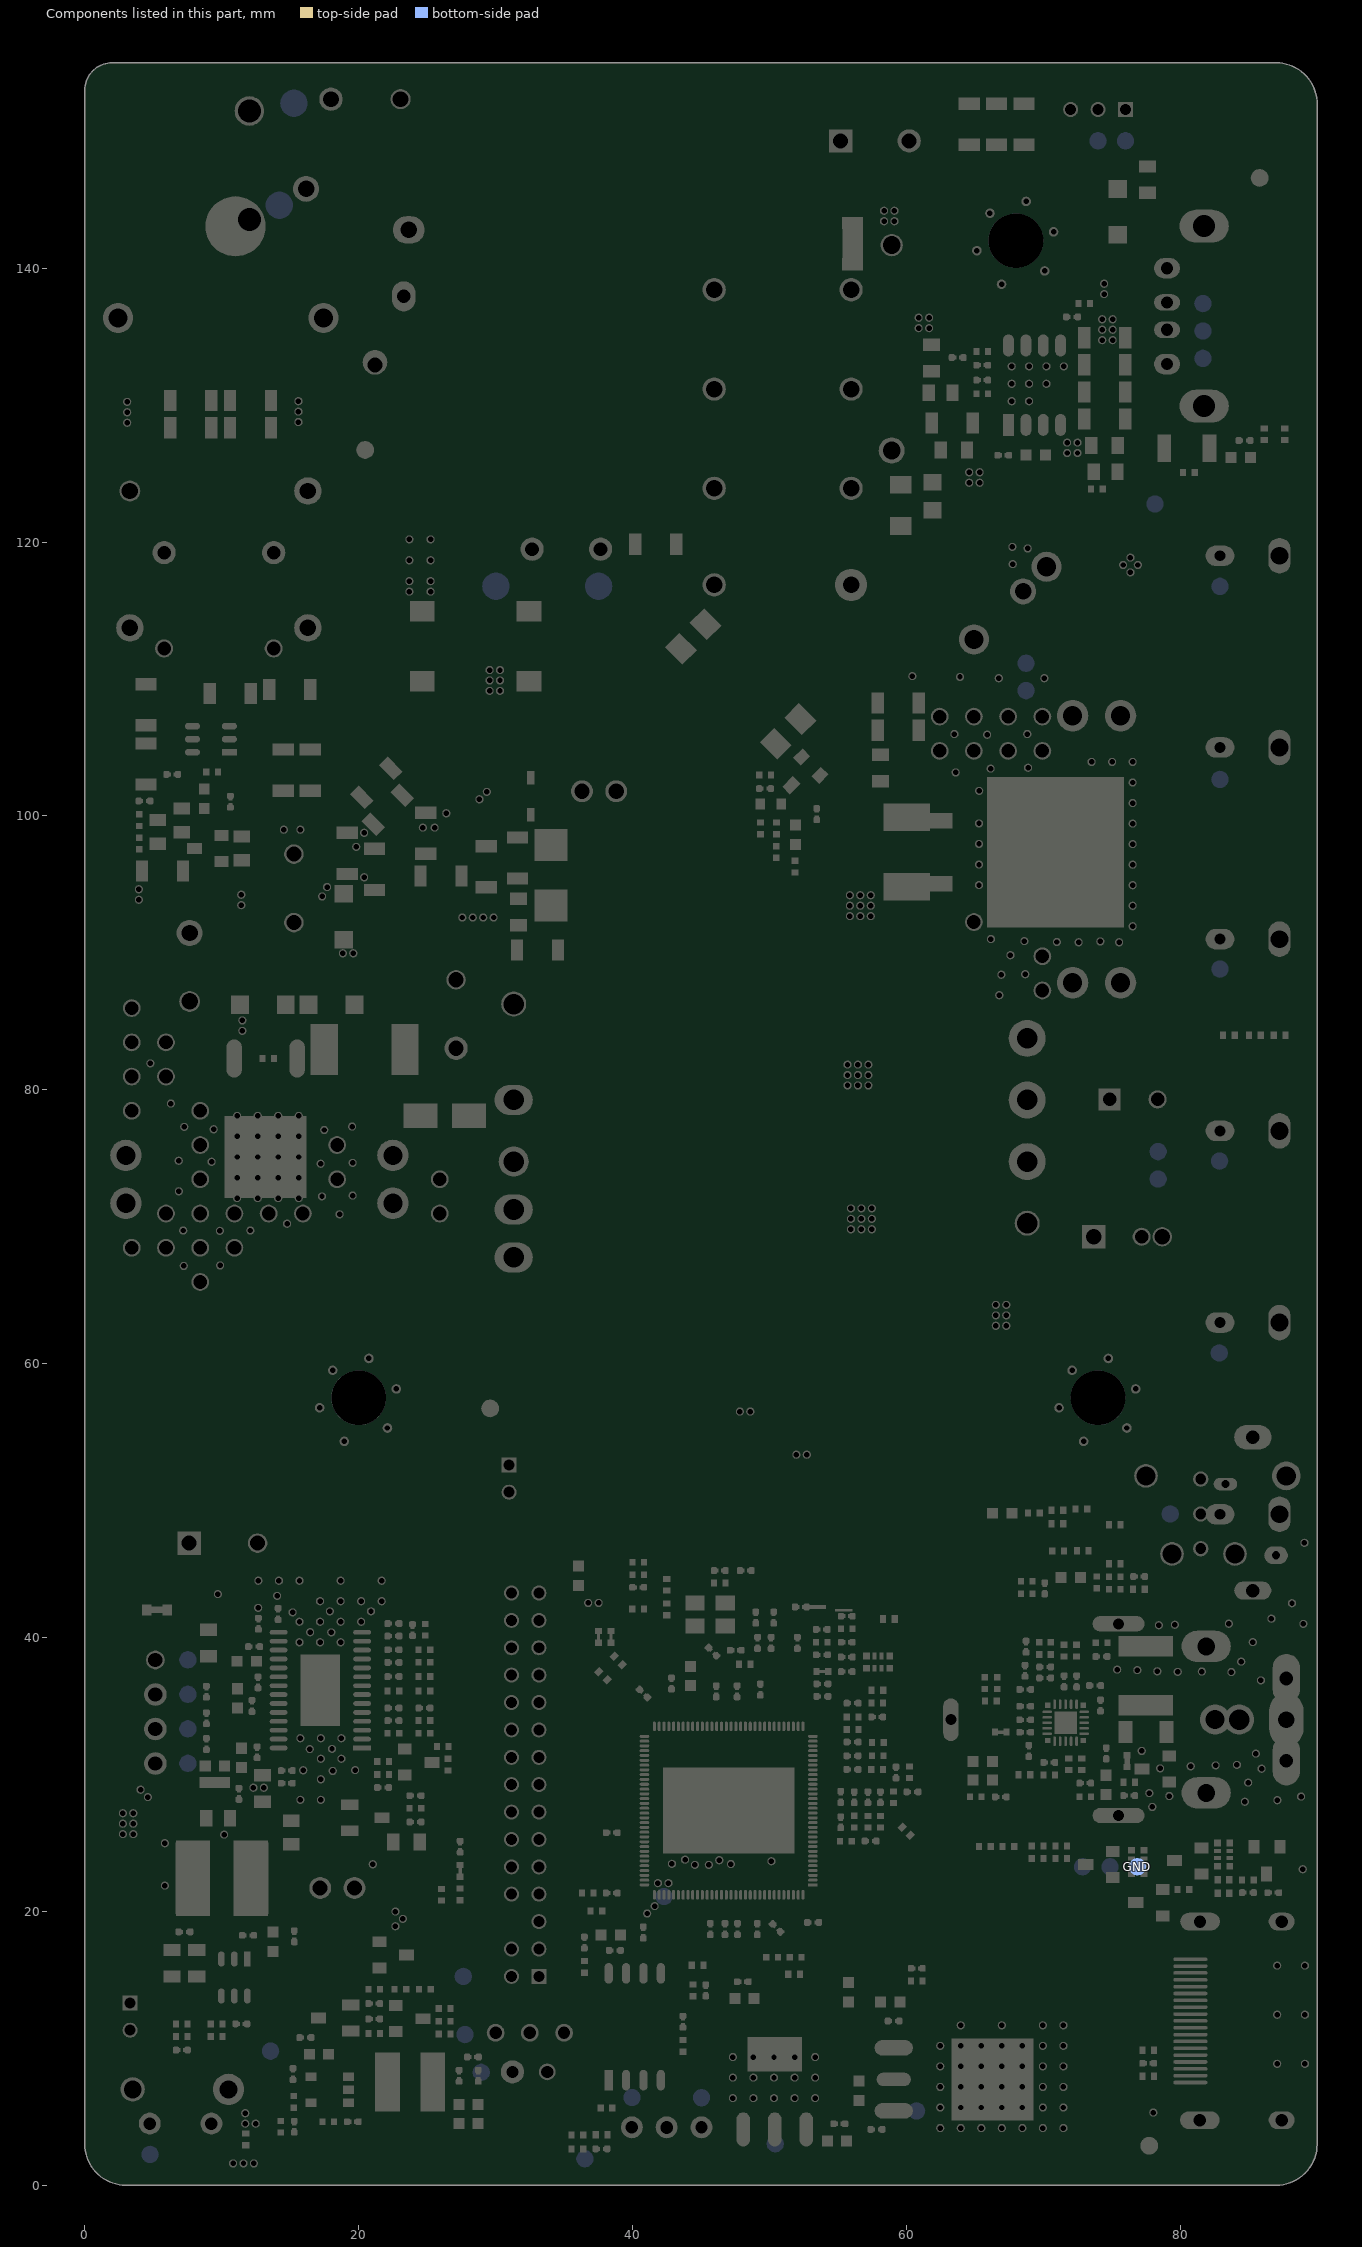
[diagram p0: the components of this part, seen from the top]
# Altium PCB MISC116569.PcbDoc (part 13 of 15)
Units mm, origin at the board's own origin, x right, y up, seen from the top; angles counter-clockwise.
Board outline 90 x 155 mm, 2 copper layers (TopLayer, BottomLayer), stack 1.571 mm thick; 527 components, 277 nets, 2450 pads, 649 vias.

## Via types
v1: diameter 0.6, hole 0.4, TopLayer to BottomLayer, tented both sides, 649 vias

## Nets (pads, with @x,y where several pads share a name; then routed paths per layer and width w, separated by ;. In a path a pad name is that pad's centre, name@x,y a point inside that pad or via, vN(x,y) a via of type N, cw(c..) or ccw(c..) an arc to the next point about the centre after c; other vN are vias at no path point) (continued)
pads on no net: "Conformal Coating.0" AV20.0 AV20.1@79.04,135.5 AV20.2@79.04,137.5 AV41.0 AV41.8 AVI1.0 AVI2.0 AVI3.0 AVO2.0 AVO3.0 AVO4.0 BOE.0 CA3.2@24.804,34.849 CA4.2@23.935,40.538 CA5.2@22.539,33.929 CA6.2@22.539,34.849 CA7.2@22.539,37.145 CA8.2@22.539,38.177 CA9.2@22.539,39.107 CA10.2@22.539,40.101 CA11.2@22.539,41.018 CA12.2@14.752,29.357 CA13.2@14.752,30.274 CA14.2@12.586,31.619 CA15.2@12.205,34.997 CA16.2@12.649,36.722 CA17.2@12.361,39.332 CA18.2@14.122,41.715 CA19.2@12.675,41.002 CA24.2@11.252,28.581 CA25.2@8.877,32.22 CA26.2@8.877,34.095 CA27.2@8.878,36.039 CA33.2@40.41,43.665 CB101.2@6.382,103.035 CB103.2@10.63,101.041 CB110.2@53.454,100.133 CB111.2@4.36,101.098 CB114.1@15.269,92.209 CB114.1@15.269,97.209 CB116.0 CB120.41 CB120.42 CB125.2@49.678,101.994 CB804.2@72.098,136.449 CB805.2@63.745,133.477 CB806.2@65.54,131.826 CB807.2@67.077,126.34 CB812.2@65.54,132.918 CD3.2@7.276,18.504 CD4.2@11.921,18.25 CD5.2@7.088,9.868 CD6.2@15.299,18.174 CD8.2@19.574,4.638 CD9.2@11.434,11.786 CD12.2@15.299,4.27 CD13.2@27.338,7.991 CD17.2@15.197,8.118 CF1.2@45.846,38.965 CF2.2@38.713,17.147 CF4.2@47.535,39.068 CF7.2@38.482,25.745 CF8.2@47.666,18.708 CF9.2@40.8,35.918 CF10.2@55.207,28.355 CF11.2@55.207,26.505 CF12.2@49.335,36.197 CF13.2@56.07,35.204 CF14.2@47.638,36.066 CF16.2@40.787,18.456 CF17.2@46.114,36.066 CF18.2@45.683,18.708 CF19.2@42.85,36.644 CF20.2@53.187,19.192 CF21.2@46.749,18.708 CF24.2@50.525,18.792 CF25.2@49.112,18.708 CF26.2@56.07,32.36 CF27.2@53.868,36.614 CF28.2@53.868,35.7 CF29.2@52.04,39.605 CF30.2@52.294,42.23 CF31.2@58.102,28.334 CF38.2@46.376,44.884 CF40.2@48.274,44.884 CG201.2@27.414,24.719 CH1.2@84.945,21.365 CH2.2@86.8,21.364 CH3.2@77.664,8.905 CH81.2@60.765,15.839 CI1.2@56.062,31.355 CI5.2@55.646,37.506 CI6.2@55.646,38.572 CI18.2@68.745,39.332 CI20.2@60.446,28.727 CI21.2@59.246,30.137 CI22.2@57.387,25.133 CK1.2@43.683,11.936 CK2.2@45.347,14.226 CK4.2@28.341,9.362 CK5.2@28.735,7.991 CK6.2@36.482,17.719 CK7.2@37.731,2.657 CL2.2@57.818,4.079 CL4.2@59.069,11.991 CL12.2@55.107,4.485 CL14.2@48.056,14.861 CM1.2@21.134,13.266 CM2.2@16.111,10.782 CM3.2@21.134,12.141 CM8.2@24.15,26.53 CM11.2@21.782,29.046 CM12.2@24.151,28.448 CN6.0 CN9.0 CNA1.0 CNA2.0 CNB1.109 CNB1.110 CNB2.0 CNB821.0 CNB831.0 CNK1.0 CNW1.0 CNW2.0 CNW2.372 CNW2.373 CNW2.374 CNW2.375 CNW2.376 CNW2.377 CNW2.378 CNW2.379 CNW2.380 CNW2.381 CNW2.382 CNW2.383 CNW2.384 CNW2.385 CNW2.386 CNW2.387 CNW2.388 CNW2.390 CNW2.391 CNW2.392 CNW2.393 CNW2.394 CNW2.395 CNW2.396 CNW2.397 CNW2.398 CNW2.400 CNW2.401 CO11.2@53.835,38.735 CO12.2@55.646,39.652 CO14.2@53.818,40.592 CO15.2@55.647,41.557 CO18.2@57.868,34.194 CO31.2@38.482,21.338 CO32.2@76.999,44.452 CO33.2@70.104,43.586 CT2.2@66.895,28.361 CT4.2@76.271,28.45 CT5.2@74.595,31.537 CT6.2@73.065,29.365 CT8.2@70.441,30.875 CT10.2@68.943,31.714 CT11.2@68.683,33.079 CT12.2@68.683,33.988 CT13.2@68.683,34.978 CT14.2@68.69,36.21 CT15.2@49.136,39.605 CT16.2@50.127,39.605 CT17.2@70.133,37.848 CT18.2@70.133,37.046 CT19.2@71.521,36.794 CT20.2@72.436,36.794 CT21.2@74.181,35.035 CT22.2@68.664,37.565 CT23.2@73.781,36.487 CT33.2@50.31,41.456 CT34.2@49.002,41.456 CT36.2@74.248,38.608 CU1.2@84.698,127.419 CV1.2@56.062,30.366 CV2.2@57.188,28.334 CV3.2@56.197,28.334 CXB1.77 CXB1.78 CYB1.61 CYB2.61 CYB3.61 CYB4.61 DB801.15 DB801.16 DK12.3 DK12.4 DK13.0 EA1.0 EB1.53 EB1.54 EB101.1@73.687,69.266 EB101.1@77.187,69.266 EB102.0 EB102.1@73.687,69.266 EB102.1@78.687,69.266 EB103.1@74.849,79.299 EB103.1@78.349,79.299 EB106.0 EB801.0 EB801.1@55.204,149.299 EB801.1@60.204,149.299 ED1.0 ED1.5 ED1.6 FB1.4 FB1.5 GD1.0 GD2.0 GD3.0 H1.0 H2.0 H3.0 HSB1.0 HSB2.0 JH1.0 LB802.1@64.94,112.893 LB802.1@70.244,118.197 LB803.3 LB803.4 LCB1.17 LCB1.18 LCB1.19 LCB1.20 LCB2.4@3.293,113.731 LCB2.4@3.293,123.731 LCB2.4@16.293,113.731 LCB2.4@16.293,123.731 M1.0 M2.0 M3.0 M4.0 Manufacture_Info.0 MOVB1.2@16.159,145.797 MOVB1.2@23.659,142.797 NTCB1.2@21.194,132.947 NTCB1.3 RFT1.0 RFT2.1@63.25,34 RFT2.1@75.5,27 RFT2.1@75.5,41 RFT2.1@87.75,34 RFT2.11 RFT3.0 RFT3.1@63.25,34 RFT3.1@75.5,27 RFT3.1@75.5,41 RFT3.3@87.75,31 RFT3.4@87.75,34 RFT3.5@87.75,37 RFT4.0 S/N1.0 S/N2.0 SK1.0 TB101.0 TB101.5 TB101.10 U1.0 U1.56 U1.59 UA1.0 UA1.13 UL2.4 UT1.1 UT1.9 UT1.10 UT1.15 XXXXXX.0 XXXXXXXXXXXXX.0 用于U1上.0
copper on no net: | length 86.4
  TopLayer w0.127: 302.535,56.174 302.535,58.174 ; 288.542,56.174 288.542,58.174 307.135,58.174 307.135,56.174 288.542,56.174
  BottomLayer w0.127: 302.535,50.641 302.535,52.641 ; 288.542,50.641 307.135,50.641 307.135,52.641 288.542,52.641 288.542,50.641

## Polygon pours and split planes (outlines as drawn)
12V on TopLayer "5" (solid, remove dead copper, pour order 1011): 63.66,116.688 60.236,116.688 59.088,115.54 59.088,105.448 64.156,100.381 64.156,92.672 63.79,92.306 65.533,90.563 65.533,84.76 65.939,84.353 68.004,84.353 70.407,81.95 70.407,81.087 73.453,78.041 74.366,78.041 74.366,80.526 77.465,83.625 77.465,115.367 75.995,116.837 71.696,116.837 69.502,114.643 65.705,114.643
D_QB101 on TopLayer "12" (solid, remove dead copper, pour order 1010): 7.798,88.303 1.341,88.303 0.541,87.503 0.541,65.608 1.24,64.91 9.715,64.91 10.058,65.253 10.058,66.256 14.3,70.498 24.587,70.498 26.251,68.834 27.076,68.834 27.635,69.393 27.635,74.917 25.743,76.81 25.743,78.486 9.576,78.486 8.103,79.959 8.103,87.998
DRIM on TopLayer "5" (solid, remove dead copper, pour order 1012): 64.13,121.285 69.07,121.285 70.683,119.672 70.683,117.196 69.744,116.256 68.791,115.303 67.699,115.303 67.267,115.303 65.349,117.221 64.422,118.148 62.962,118.148 59.418,118.148 59.317,118.25 60.117,119.05 60.117,120.51 60.117,120.612 60.295,120.79
NetBB801_2 on TopLayer "5" (solid, remove dead copper, pour order 1013): 59.749,128.105 59.749,127.394 59.787,127.356 62.886,127.356 63.025,127.216 63.025,124.282 62.632,123.888 58.352,123.888 57.933,124.308 57.933,127.61 58.631,128.308 59.139,128.308
GND on TopLayer "5" (solid, remove dead copper, pour order 1018): 53.581,24.748 53.581,22.438 53.075,21.932 52.504,21.361 52.256,21.361 52.256,20.551 52.09,20.386 52.524,19.953 53.157,19.953 54.376,19.953 56.053,18.275 57.976,16.352 60.801,16.352 71.768,16.352 76.716,11.405 77.314,10.806 78.049,10.806 78.545,10.311 79.144,10.311 79.333,10.5 79.349,10.516 79.434,10.516 79.434,17.462 79.357,17.539 78.122,17.539 75.666,19.995 74.043,21.618 69.363,21.618 61.933,21.618 61.463,22.088 60.529,22.088 60.288,22.328 60.033,22.073 59.533,22.073 59.461,22.073 57.598,23.935 57.191,24.342 54.584,24.342 54.186,24.74 54.072,24.854 53.856,24.854 53.687,24.854 53.581,24.748
GND on TopLayer "5" (solid, remove dead copper, pour order 1021): 47.078,34.29 41.309,34.29 40.527,33.508 40.527,23.247 42.032,21.742 51.519,21.742 52.497,22.72 52.497,32.41 51.399,33.508 47.974,33.508 47.078,34.404
GND on TopLayer "5" (solid, remove dead copper, pour order 1020): 30.742,44.31 30.221,43.79 30.221,43.624 30.221,20.127 29.084,18.99 29.156,18.918 29.251,18.918 29.366,18.918 30.056,19.609 30.668,20.221 33.104,20.221 33.722,20.221 34.943,21.442 34.943,22.017 35.902,22.977 37.333,22.977 39.79,22.977 40.33,23.517 40.483,23.67 40.483,27.33 40.483,32.979 40.709,33.205 41.011,33.508 42.299,33.508 42.299,34.866 41.548,35.617 41.101,35.617 41.101,36.365 40.389,37.077 40.389,38.067 39.7,38.756 39.7,41.425 39.981,41.707 39.981,42.078 39.568,42.491 38.262,42.491 38.113,42.342 38.113,42 37.619,41.506 36.56,41.506 36.244,41.822 33.69,44.376 31.707,44.376 30.808,44.376 30.742,44.31
GND on TopLayer "12" (solid, remove dead copper, pour order 1019): 22.474,61.316 2.489,61.316 0,58.826 0,1.227 0.77,0.457 1.227,0 3.907,0 88.603,0 89.352,0.749 90.009,1.406 90.009,3.137 90.009,52.36 89.469,52.9 30.844,52.9 22.5,61.244
GND on TopLayer "12" (solid, remove dead copper, pour order 1008): 68.999,147.523 65.697,147.523 64.579,146.406 63.03,144.856 63.03,144.729 62.7,144.399 62.7,141.135 62.7,139.649 64.872,137.477 65.824,136.525 69.507,136.525 70.244,136.525 72.136,138.417 73.254,139.535 73.254,143.586 73.254,144.666 71.971,145.948 70.396,147.523 69.393,147.523
GND on TopLayer "12" (solid, remove dead copper, pour order 1009): 69.659,134.29 69.659,133.502 69.393,133.236 67.539,133.236 66.827,132.524 66.827,130.442 67.45,129.819 71.526,129.819 71.996,130.289 71.996,132.766 71.615,133.147 70.777,133.147 70.358,133.566 70.358,134.252 69.952,134.658
GND on TopLayer "12" (solid, remove dead copper, pour order 1003): 86.831,45.098 86.831,52.107 85.128,53.81 85.128,54.813 87.135,56.82 87.859,57.544 87.859,60.706 87.859,82.563 88.328,83.033 88.328,84.442 87.643,85.128 87.643,117.107 86.97,117.78 86.093,118.656 86.093,122.047 86.093,122.923 87.909,124.739 88.887,125.717 88.887,128.27 88.887,136.627 87.63,137.884 81.826,137.884 81.089,138.62 81.089,141.719 80.15,142.659 80.15,154.368 80.861,155.08 88.201,155.08 89.611,153.67 90,153.281 90,152.003 90,44.443 89.469,43.912
GND on TopLayer "5" (solid, remove dead copper, pour order 1005): 80.708,137.414 85.966,137.414 87.363,136.017 87.884,135.496 87.884,134.341 87.884,129.153 88.332,128.705 88.332,127.732 87.6,127 87.6,126.087 86.388,124.875 81.402,119.89 81.402,117.399 81.402,88.587 82.169,87.82 82.169,81.829 81.402,81.062 81.402,80.15 81.402,74.04 82.18,73.263 83.109,72.334 83.109,68.732 83.109,66.197 81.733,64.821 81.212,64.3 81.212,61.76 81.212,57.051 81.212,54.879 80.524,54.192 79.621,53.288 79.621,52.591 79.621,50.627 78.702,49.708 78.217,49.223 76.517,49.223 76.517,49.708 76.253,49.972 75.937,50.288 74.016,50.288 40.084,50.288 39.357,49.561 39.357,37.335 39.453,37.239 38.588,37.239 36.787,39.04 36.584,39.243 36.584,39.294 36.584,40.471 37.93,41.817 37.998,41.885 37.998,42.922 37.998,50.393 39.141,51.537 39.459,51.854 41.554,51.854 76.271,51.854 76.367,51.759 76.367,51.383 76.708,51.041 77.003,50.746 77.937,50.746 78.554,51.363 78.554,52.434 78.168,52.819 78.168,53.835 79.438,55.105 79.713,55.38 79.713,56.985 79.713,64.92 81.61,66.818 81.61,67.805 81.61,71.713 79.904,73.42 79.904,74.536 79.904,81.683 80.704,82.483 80.704,86.968 79.904,87.768 79.904,88.811 79.904,120.645 84.315,125.057 86.117,126.859 86.117,127.451 85.555,128.014 85.555,128.626 86.101,129.172 86.101,133.837 85.89,134.048 81.521,134.048 81.204,134.366 81.204,135.664 81.496,135.956 81.496,136.627 80.708,137.414
GND on TopLayer "12" (solid, remove dead copper, pour order 1007): 74.816,62.357 72.123,62.357 70.65,60.884 69.393,59.627 69.393,58.75 69.393,55.385 69.964,54.813 71.793,52.984 72.276,52.984 76.302,52.984 77.025,53.708 78.562,55.245 78.562,56.21 78.562,59.639 77.851,60.35 75.781,62.42 74.562,62.42
L on TopLayer "12" (solid, remove dead copper, pour order 1002): 15.095,114.719 13.14,112.763 13.14,112.159 13.729,111.569 14.999,111.569 15.799,110.769 15.799,108.61 15.938,108.471 16.904,108.471 17.361,108.928 17.463,109.029 25.4,109.029 25.662,109.291 25.662,110.68 25.281,111.061 20.98,111.061 17.323,114.719
N-3 on TopLayer "5" (solid, remove dead copper, pour order 1017): 2.307,109.283 2.41,109.18 5.225,109.18 5.253,109.208 5.253,110.765 6.464,111.976 6.464,113.317 4.821,114.96 2.954,114.96 2.307,114.313
SGND on BottomLayer "12" (solid, remove dead copper, pour order 1006): 11.551,103.672 9.654,103.672 9.19,103.208 7.175,103.208 7.175,102.441 5.08,100.346 4.931,100.346 3.81,99.225 3.81,95.936 4.851,94.894 10.071,94.894 10.935,94.031 10.935,93.345 11.138,93.142 11.671,93.142 11.925,93.396 11.925,94.463 10.49,95.898 6.299,95.898 5.601,96.596 5.601,98.848 6.524,99.771 10.071,99.771 10.211,99.911 10.211,100.495 10.071,100.635 9.296,100.635 9.106,100.825 9.106,101.473 9.817,102.184 10.465,102.184 11.582,103.302 11.582,103.64
GND on BottomLayer "12" (solid, remove dead copper, pour order 1000): 73.063,145.961 76.962,145.961 78.956,147.955 78.956,154.52 79.438,155.003 88.736,155.003 89.484,154.254 90,153.738 90,152.003 90,142.641 87.427,140.068 78.257,140.068 75.882,142.443 74.511,143.815 73.812,143.815
D_QB101 on BottomLayer "12" (solid, remove dead copper, pour order 1001): 1.422,87.389 0.541,86.508 0.541,65.608 1.24,64.91 9.05,64.91 9.609,65.468 9.609,65.845 12.344,68.58 12.548,68.58 13.487,69.52 14.059,69.52 16.485,70.421 20.333,70.828 23.812,70.218 26.251,69.113 26.429,68.936 27.8,68.936 27.8,78.143 27.267,78.676 11.176,78.676 8.534,81.318 8.534,86.893 8.039,87.389
GND on BottomLayer "5" (solid, remove dead copper, pour order 1016): 62.873,136.639 62.873,127.787 64.308,126.352 69.286,126.352 69.744,126.809 69.744,130.564 70.739,131.559 75.019,131.559 75.56,132.101 75.56,138.481 74.912,139.129 73.896,139.129 70.607,135.839 64.003,135.839 63.292,136.55
GND on BottomLayer "12" (solid, remove dead copper, pour order 1014): 23.762,66.51 19.164,61.912 2.261,61.912 -0.076,59.576 -0.076,1.245 1.168,0 88.697,0 90.009,1.312 90.009,143.836 89.37,144.475 79.883,144.475 77.495,146.863 73.558,146.863 71.476,148.946 64.706,148.946 63.208,147.447 63.208,139.497 65.697,137.008 70.371,137.008 73.406,140.043 75.324,140.043 76.187,139.179 76.187,130.404 75.679,129.896 75.679,120.523 79.28,116.922 79.28,82.155 78.601,81.476 78.601,67.755 78.054,67.208 61.988,67.208 61.01,66.23 45.555,66.23 36.83,57.506 26.835,57.506 22.425,61.916 19.122,61.916
GND on BottomLayer "5" (solid, remove dead copper, pour order 1004): 53.53,62.014 44.869,62.014 35.827,52.972 33.287,50.432 33.287,49.2 21.031,49.2 20.51,48.679 20.51,24.27 22.212,22.568 23.546,21.234 23.546,20.574 23.546,20.206 24.219,19.533 24.295,19.456 24.295,18.732 24.295,16.423 24.589,16.129 24.69,16.027 31.191,16.027 32.048,16.027 32.22,16.199 32.22,18.961 34.265,21.006 35.001,20.269 35.001,14.694 35.001,13.437 36.551,11.887 39.192,9.246 42.227,9.246 43.917,9.246 46.571,11.9 57.302,11.9 60.16,14.757 65.164,19.761 84.176,19.761 84.176,28.346 79.096,33.426 72.403,40.119 72.403,48.273 68.021,48.273 53.53,62.763
12V on BottomLayer "5" (solid, remove dead copper, pour order 1015): 62.865,115.951 55.748,108.834 55.748,101.122 59.571,97.3 59.571,83.749 60.617,82.702 65.629,82.702 67.661,84.734 73.884,84.734 76.995,87.846 76.995,112.662 75.852,113.805 67.445,113.805 65.299,115.951

## Keep-outs
KeepOutLayer:
  rectangle: 288.542,41.003 291.849,43.003
  lines w0.127: 302.535,41.003 302.535,43.003 ; 87,155.003 cw(c87,152.003) 90,152.003 90,3 cw(c87,3) 87,0 3,0 cw(c3,3) 0,3 0,153.003 cw(c2,153.003) 2,155.003 87,155.003 ; 87,155.003 ccw(c87,158.003) 90,158.003 90,307.005 ccw(c87,307.005) 87,310.005 2,310.005 ccw(c2,308.005) 0,308.005 0,158.003 ccw(c3,158.003) 3,155.003 87,155.003 ; 93.009,155.003 ccw(c93.009,152.003) 90.009,152.003 90.009,3 ccw(c93.009,3) 93.009,0 178.009,0 ccw(c178.009,2) 180.009,2 180.009,152.003 ccw(c177.009,152.003) 177.009,155.003 93.009,155.003 ; 93.009,155.003 cw(c93.009,158.003) 90.009,158.003 90.009,307.005 cw(c93.009,307.005) 93.009,310.005 177.009,310.005 cw(c177.009,307.005) 180.009,307.005 180.009,157.003 cw(c178.009,157.003) 178.009,155.003 93.009,155.003 ; 288.542,41.003 307.135,41.003 307.135,43.003 288.542,43.003 288.542,41.003
  lines w1.2: 67.998,136.986 ccw(c67.864,142.004) 72.432,139.923
  text "KeepOutLayer" at 292.423,41.536 h1.52
  text ".GKO" at 303.137,41.462 h1.52

## Other copper
TopLayer:
  drawing of 291 lines, arcs and shapes, not listed
  text "TopLayer" at 292.759,56.742 h1.52
  text ".GTL" at 303.16,56.633 h1.52